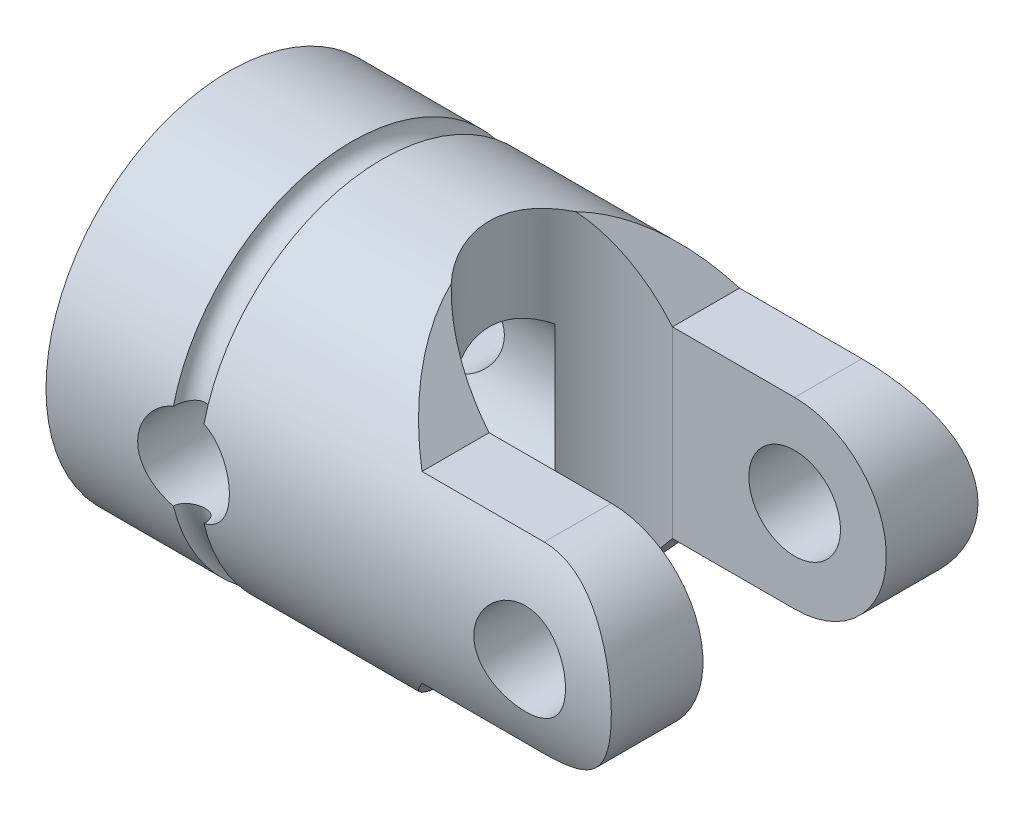
from build123d import *

# Parameters (mm, degrees)
CUT_EXTRUDE_1_DEPTH      = 21.353132437
CUT_EXTRUDE_1_DEPTH_BACK = 21.353132437
CUT_EXTRUDE_2_DEPTH      = 21.353132587
CUT_EXTRUDE_2_DEPTH_BACK = 21.353132587
SKETCH_2_R               = 3


with BuildPart() as part:
    # 草图1 one side → 旋转3 (revolve)
    with BuildSketch(Plane.XY, mode=Mode.PRIVATE) as revolve_3_sk:
        with BuildLine():
            Line((18.5, 0), (18.5, 6))
            Line((18.5, 6), (5, 6))
            ThreePointArc((5, 6), (4.5, 5.5), (4, 6))
            Line((4, 6), (0, 6))
            Line((0, 6), (0, 3))
            Line((0, 3), (9, 3))
            Line((9, 3), (9, 0))
            Line((9, 0), (14, 0))
            ThreePointArc((14, 0), (15.5, 1.5), (17, 0))
            Line((17, 0), (18.5, 0))
        make_face()
    revolve(revolve_3_sk.sketch.rotate(Axis((0, 0, 0), (1, 0, 0)), 90), axis=Axis((0, 0, 0), (1, 0, 0)))

    # 草图1<11> → 切除-拉伸1 (cut, two sides: drawn at the far end of the back side and taken through both)
    with BuildSketch(Plane.XY.offset(-CUT_EXTRUDE_1_DEPTH_BACK)):
        with BuildLine():
            Line((11.5, 3), (15.5, 3))
            ThreePointArc((15.5, 3), (17.621320344, 2.121320344), (18.5, 0))
            Line((18.5, 0), (18.5, 6))
            Line((18.5, 6), (9, 6))
            Line((9, 6), (11.5, 3))
        make_face()
        with BuildLine():
            Line((18.5, -6), (18.5, 0))
            ThreePointArc((18.5, 0), (17.621320344, -2.121320344), (15.5, -3))
            Line((15.5, -3), (11.5, -3))
            Line((11.5, -3), (9, -6))
            Line((9, -6), (18.5, -6))
        make_face()
        with BuildLine():
            ThreePointArc((14, 0), (15.5, -1.5), (17, 0))
            Line((17, 0), (14, 0))
        make_face()
        with BuildLine():
            Line((14, 0), (17, 0))
            ThreePointArc((17, 0), (15.5, 1.5), (14, 0))
        make_face()
        with BuildLine():
            ThreePointArc((3, 0), (4.5, -1.5), (6, 0))
            Line((6, 0), (3, 0))
        make_face()
        with BuildLine():
            Line((3, 0), (6, 0))
            ThreePointArc((6, 0), (4.5, 1.5), (3, 0))
        make_face()
        with BuildLine():
            ThreePointArc((3, 0), (4.5, -1.5), (6, 0))
            Line((6, 0), (3, 0))
        make_face()
        with BuildLine():
            Line((3, 0), (6, 0))
            ThreePointArc((6, 0), (4.5, 1.5), (3, 0))
        make_face()
        with BuildLine():
            ThreePointArc((14, 0), (15.5, -1.5), (17, 0))
            Line((17, 0), (14, 0))
        make_face()
        with BuildLine():
            Line((14, 0), (17, 0))
            ThreePointArc((17, 0), (15.5, 1.5), (14, 0))
        make_face()
    extrude(amount=CUT_EXTRUDE_1_DEPTH + CUT_EXTRUDE_1_DEPTH_BACK, mode=Mode.SUBTRACT)

    # 草图2 → 切除-拉伸2 (cut, two sides: drawn at the far end of the back side and taken through both)
    with BuildSketch(Plane(origin=(0, 0, 0), x_dir=(1, 0, 0), z_dir=(0, 1, 0)).offset(-CUT_EXTRUDE_2_DEPTH_BACK)):
        with Locations((11.5, 0)):
            Circle(SKETCH_2_R)
        with BuildLine():
            Line((18.5, 3), (11.5, 3))
            ThreePointArc((11.5, 3), (13.621320344, 2.121320344), (14.5, 0))
            ThreePointArc((14.5, 0), (13.621320344, -2.121320344), (11.5, -3))
            Line((11.5, -3), (18.5, -3))
            Line((18.5, -3), (18.5, 3))
        make_face()
    extrude(amount=CUT_EXTRUDE_2_DEPTH + CUT_EXTRUDE_2_DEPTH_BACK, mode=Mode.SUBTRACT)


solid = part.part
